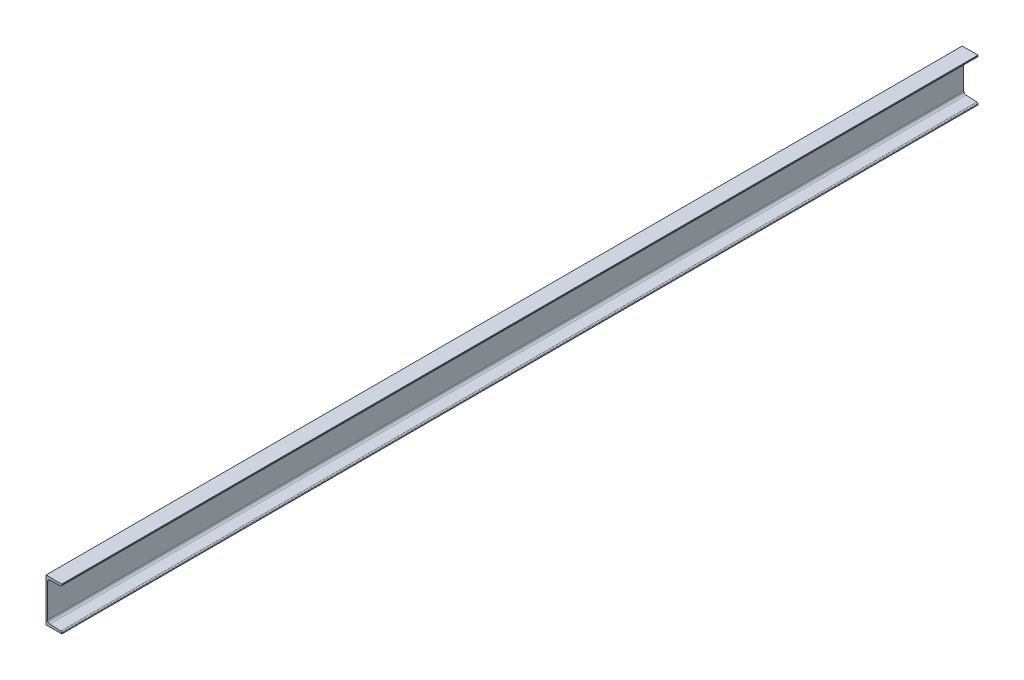
from build123d import *

# Parameters (mm, degrees)
BOSS_EXTRUDE1_DEPTH = 2120.9


with BuildPart() as part:
    # Sketch1 → Boss-Extrude1 (new, symmetric)
    with BuildSketch(Plane(origin=(28.211262136, 0, 0), x_dir=(-1, 0, 0), z_dir=(0, 0, 1))):
        with BuildLine():
            Line((28.211262136, 0), (28.211262136, -200))
            Line((28.211262136, -200), (-44.788737864, -200))
            Line((-44.788737864, -200), (-44.788737864, -196.033179359))
            ThreePointArc((-44.788737864, -196.033179359), (-43.272315441, -192.240936001), (-39.559243433, -190.539835501))
            Line((-39.559243433, -190.539835501), (10.752273273, -188.062374452))
            ThreePointArc((10.752273273, -188.062374452), (18.17841729, -184.660173452), (21.211262136, -177.075686736))
            Line((21.211262136, -177.075686736), (21.211262136, -22.924313264))
            ThreePointArc((21.211262136, -22.924313264), (18.17841729, -15.339826548), (10.752273273, -11.937625548))
            Line((10.752273273, -11.937625548), (-39.559243433, -9.460164499))
            ThreePointArc((-39.559243433, -9.460164499), (-43.272315441, -7.759063999), (-44.788737864, -3.966820641))
            Line((-44.788737864, -3.966820641), (-44.788737864, 0))
            Line((-44.788737864, 0), (28.211262136, 0))
        make_face()
    extrude(amount=BOSS_EXTRUDE1_DEPTH, both=True)


solid = part.part
